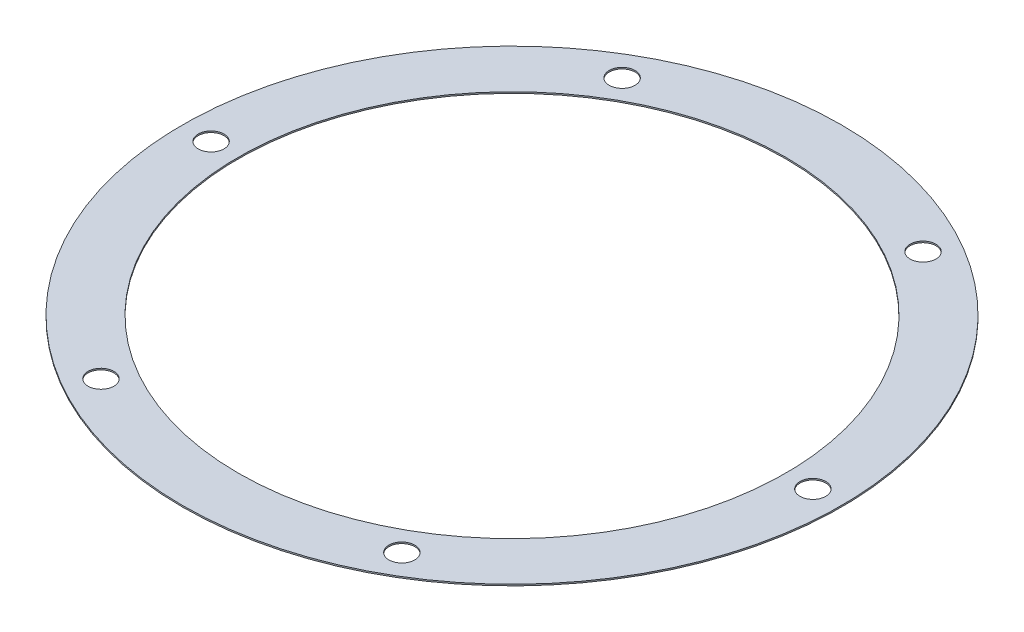
SolidWorks part; units mm, degrees
material "XB150"
ref_plane "Front Plane" through (0, 0, 0) normal (0, 0, 1) x (1, 0, 0)
ref_plane "Top Plane" through (0, 0, 0) normal (0, 1, 0) x (1, 0, 0)
ref_plane "Right Plane" through (0, 0, 0) normal (1, 0, 0) x (0, 0, -1)
sketch "Sketch1" plane through (0, 0, 0) normal (0, 1, 0) x (1, 0, 0)
  line L0 (-286.0405, 0) -> (286.0405, 0) construction
  line L1 (0, 241.9011) -> (0, -262.6726) construction
  circle A0 centre (0, 0) radius 230
  circle A1 centre (0, 0) radius 191
  dimension "D1" = 460
  dimension "D2" = 382
extrude "Boss-Extrude1" add sketch "Sketch1" along normal mid plane 1
sketch "Sketch2" plane through (0, 0, 0) normal (0, 1, 0) x (1, 0, 0)
  line L0 (0, 0) -> (-267.5282, 0) construction
  circle A0 centre (0, 0) radius 210 construction
  circle A1 centre (-210, 0) radius 9
  dimension "D1" = 420
  dimension "D2" = 18
extrude "Cut-Extrude2" cut sketch "Sketch2" along normal mid plane 1
pattern_circular "CirPattern1" count 6 over 360 about axis through (0, 0, 0) along (0, 1, 0) of "Cut-Extrude2"
